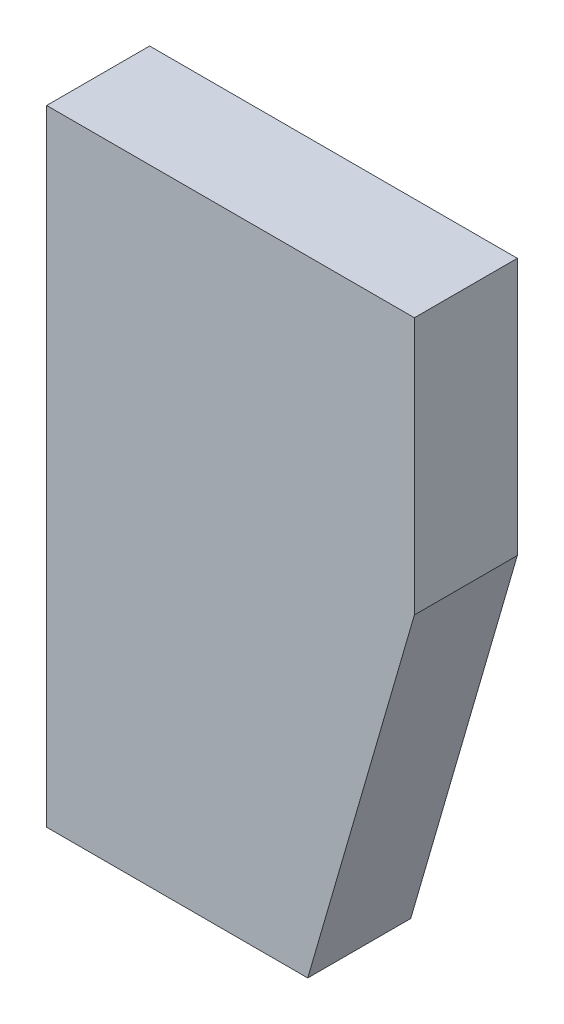
from build123d import *

# Parameters (mm, degrees)
EXTRUDE_1_DEPTH = 14


with BuildPart() as part:
    # 草图1 → 凸台-拉伸1 (new body)
    with BuildSketch(Plane.XY):
        Polygon((0, 0), (0, 85), (50, 85), (50, 50), (35.5, 0), align=None)
    extrude(amount=EXTRUDE_1_DEPTH)


solid = part.part
